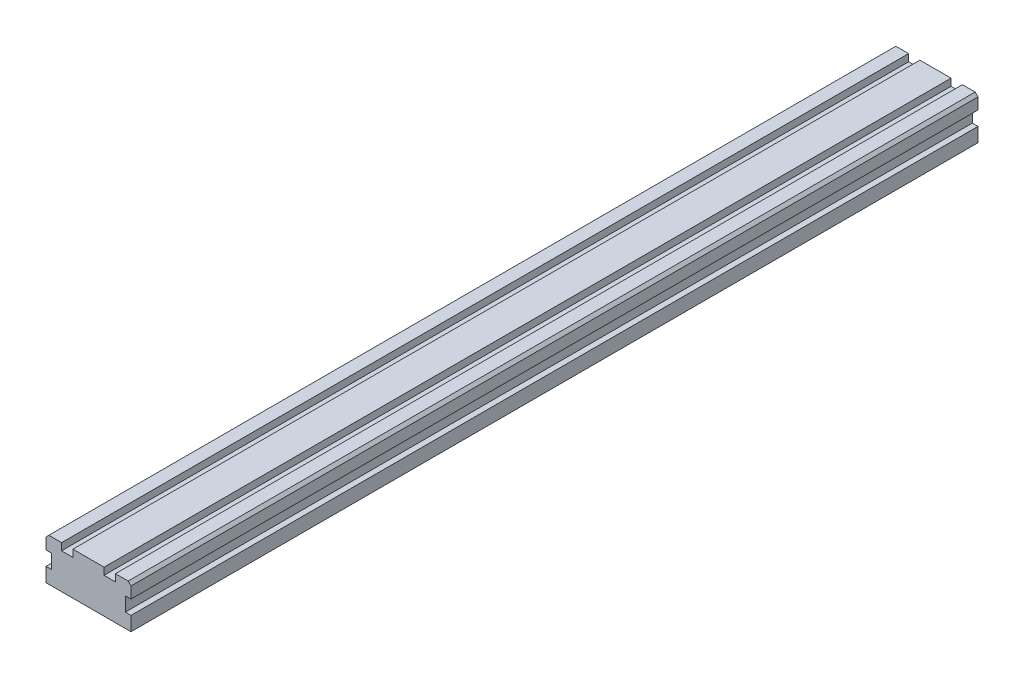
SolidWorks part; units mm, degrees
ref_plane "Front Plane" through (0, 0, 0) normal (0, 0, 1) x (1, 0, 0)
ref_plane "Top Plane" through (0, 0, 0) normal (0, 1, 0) x (1, 0, 0)
ref_plane "Right Plane" through (0, 0, 0) normal (1, 0, 0) x (0, 0, -1)
sketch "Sketch1" plane through (0, 0, 0) normal (0, 0, 1) x (1, 0, 0)
  line L0 (720, 30) -> (720, 45) construction
  line L1 (735, 30) -> (705, 30) construction
  line L3 (750, 60) -> (690, 60)
  line L4 (750, 60) -> (750, 30)
  line L5 (750, 30) -> (690, 30)
  line L6 (690, 60) -> (690, 30)
  line L7 (750, 60) -> (690, 30) construction
  line L8 (750, 30) -> (690, 60) construction
  dimension "D1" = 60
  dimension "D2" = 30
extrude "Boss-Extrude1" add sketch "Sketch1" along normal mid plane 598
sketch "Sketch2" plane through (0, 0, -299) normal (0, 0, -1) x (-1, 0, 0)
  line L0 (-750, 60) -> (-690, 60) construction
  line L1 (-739, 65) -> (-731, 65)
  line L2 (-739, 65) -> (-739, 55)
  line L3 (-739, 55) -> (-731, 55)
  line L4 (-731, 65) -> (-731, 55)
  line L5 (-739, 65) -> (-731, 55) construction
  line L6 (-739, 55) -> (-731, 65) construction
  line L7 (-720, 60) -> (-720, 42.968) construction
  line L8 (-750, 30) -> (-750, 60) construction
  line L9 (-754, 50) -> (-746, 50)
  line L10 (-754, 50) -> (-754, 40)
  line L11 (-754, 40) -> (-746, 40)
  line L12 (-746, 50) -> (-746, 40)
  line L13 (-754, 50) -> (-746, 40) construction
  line L14 (-754, 40) -> (-746, 50) construction
  line L15 (-686, 40) -> (-694, 50) construction
  line L16 (-686, 50) -> (-694, 40) construction
  line L17 (-701, 55) -> (-709, 65) construction
  line L18 (-701, 65) -> (-709, 55) construction
  line L19 (-694, 50) -> (-694, 40)
  line L20 (-686, 40) -> (-694, 40)
  line L21 (-686, 50) -> (-686, 40)
  line L22 (-686, 50) -> (-694, 50)
  line L23 (-709, 65) -> (-709, 55)
  line L24 (-701, 55) -> (-709, 55)
  line L25 (-701, 65) -> (-701, 55)
  line L26 (-701, 65) -> (-709, 65)
  point P0 (-735, 60)
  point P9 (-750, 45)
  point P24 (-690, 45)
  point P25 (-705, 60)
  dimension "D1" = 11
  dimension "D2" = 10
  dimension "D3" = 8
  dimension "D4" = 10
  dimension "D5" = 8
extrude "Cut-Extrude1" cut sketch "Sketch2" against normal blind 646
chamfer "Chamfer1" distance 2 angle 45 2 edges at (690, 60, 0) (750, 60, 0)
